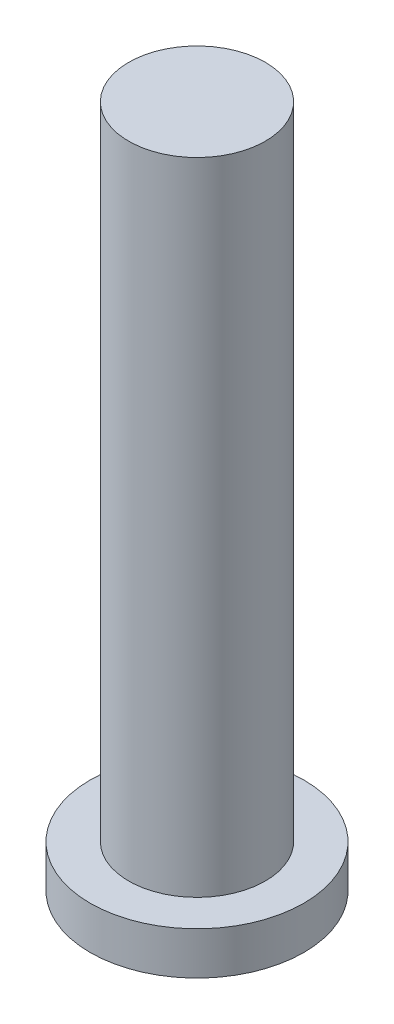
SolidWorks part; units mm, degrees
ref_plane "前视基准面" through (0, 0, 0) normal (0, 0, 1) x (1, 0, 0)
ref_plane "上视基准面" through (0, 0, 0) normal (0, 1, 0) x (1, 0, 0)
ref_plane "右视基准面" through (0, 0, 0) normal (1, 0, 0) x (0, 0, -1)
sketch "草图1" plane through (0, 0, 0) normal (0, 0, 1) x (1, 0, 0)
  line L0 (0, 0) -> (4, 0)
  line L1 (4, 0) -> (4, -37.5)
  line L2 (4, -37.5) -> (6.25, -37.5)
  line L3 (6.25, -37.5) -> (6.25, -40)
  line L4 (6.25, -40) -> (0, -40)
  line L5 (0, -40) -> (0, 0)
  dimension "D1" = 6.25
  dimension "D2" = 4
  dimension "D3" = 2.5
  dimension "D4" = 40
revolve "旋转1" add sketch "草图1" angle 360 about L5
